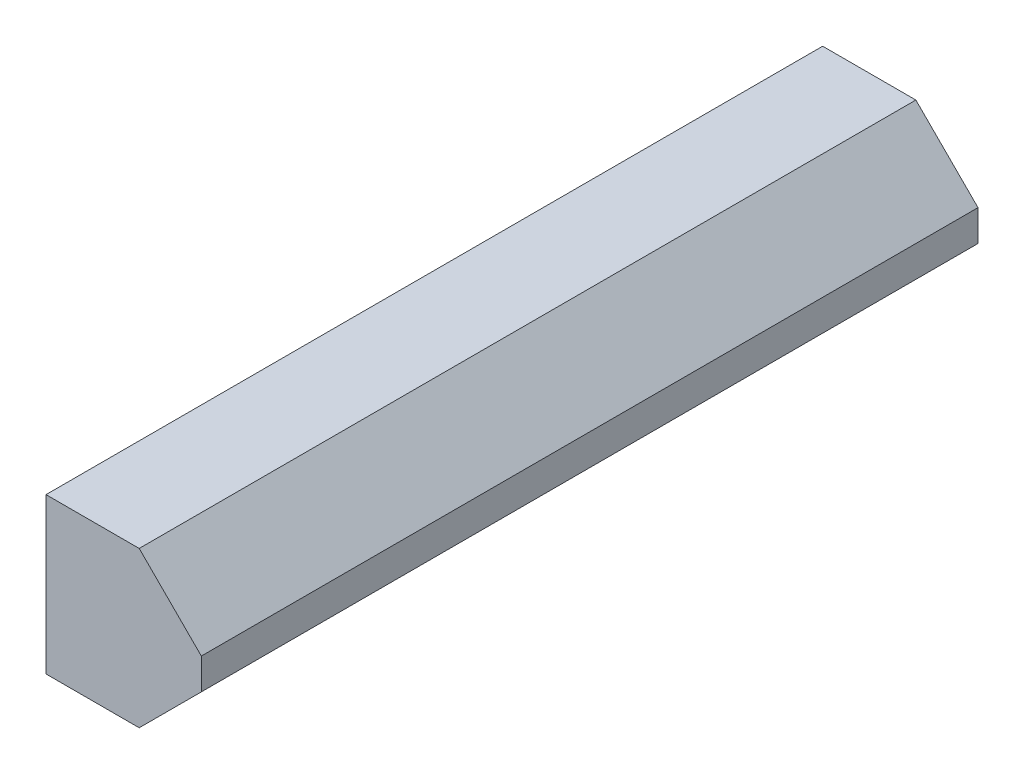
from build123d import *

# Parameters (mm, degrees)
SKETCH1_W           = 250
SKETCH1_H           = 50
BOSS_EXTRUDE1_DEPTH = 25
CHAMFER1_SIZE       = 20


with BuildPart() as part:
    # Sketch1 → Boss-Extrude1 (new, symmetric)
    with BuildSketch(Plane(origin=(0, 0, 0), x_dir=(0, 0, -1), z_dir=(1, 0, 0))):
        Rectangle(SKETCH1_W, SKETCH1_H)
    extrude(amount=BOSS_EXTRUDE1_DEPTH, both=True)

    # Chamfer1
    chamfer1_edges = [part.edges().sort_by_distance(p)[0] for p in [
        (25, 25, 0),
        (25, -25, 0),
    ]]
    chamfer(chamfer1_edges, length=CHAMFER1_SIZE)


solid = part.part
